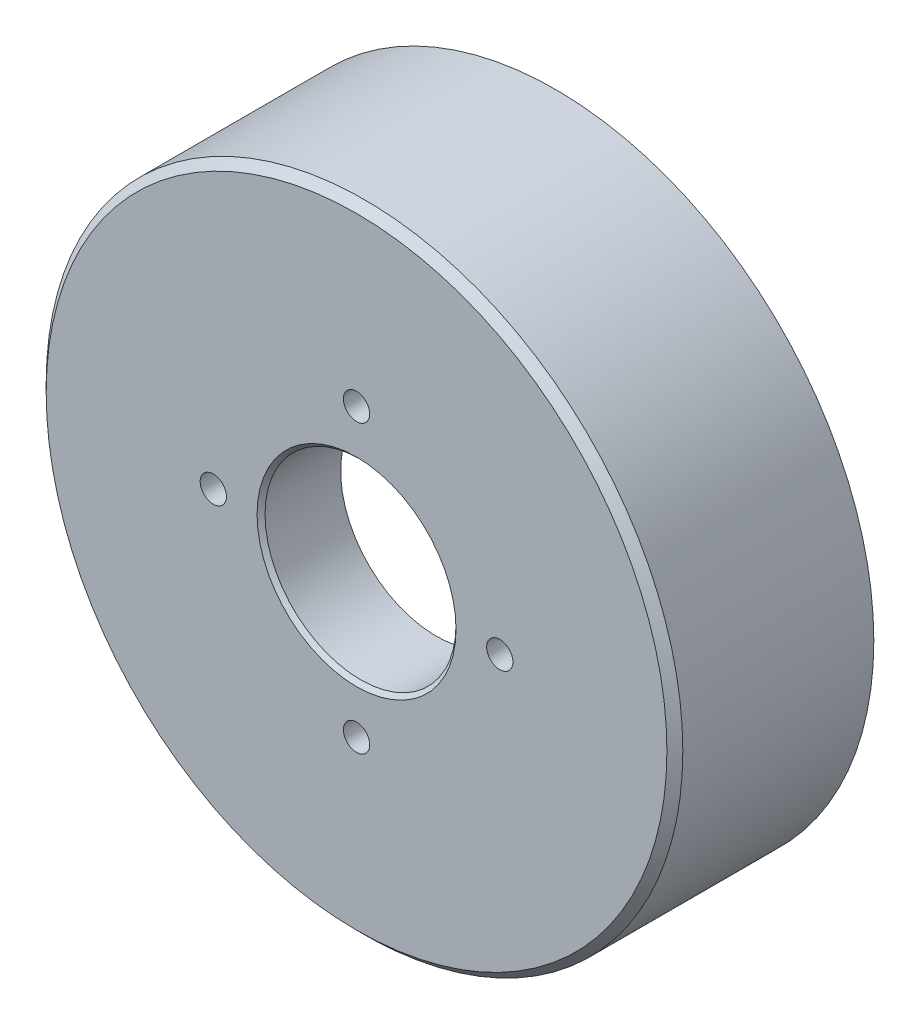
from build123d import *

# Parameters (mm, degrees)
CHAMFER1_SIZE      = 1
SKETCH9_R          = 12
CUT_EXTRUDE1_DEPTH = 62.846584384
M4_TAPPED_HOLE1_D  = 3.3
CHAMFER2_SIZE      = 0.5


with BuildPart() as part:
    # Sketch8 → Revolve2 (revolve)
    with BuildSketch(Plane(origin=(0, 0, 0), x_dir=(0, 0, -1), z_dir=(1, 0, 0)), mode=Mode.PRIVATE) as revolve2_sk:
        Polygon((0, 0), (0, 40), (25, 40), (25, 35), (10, 35), (10, 0), align=None)
    revolve(revolve2_sk.sketch.rotate(Axis((0, 0, 0), (0, 0, -1)), 90), axis=Axis((0, 0, 0), (0, 0, -1)))

    # Chamfer1
    chamfer1_edges = [part.edges().sort_by_distance(p)[0] for p in [
        (-40, 0, 0),
    ]]
    chamfer(chamfer1_edges, length=CHAMFER1_SIZE)

    # Sketch9 → Cut-Extrude1 (cut, through all)
    with BuildSketch(Plane.XY):
        Circle(SKETCH9_R)
    extrude(amount=-CUT_EXTRUDE1_DEPTH, mode=Mode.SUBTRACT)

    # M4 Tapped Hole1 (through all)
    with Locations(Plane(origin=(0, 18, 0), x_dir=(1, 0, 0), z_dir=(0, 0, 1))):
        with Locations((0, 0), (-18, -18), (18, -18), (0, -36)):
            Hole(M4_TAPPED_HOLE1_D / 2)

    # Chamfer2
    chamfer2_edges = [part.edges().sort_by_distance(p)[0] for p in [
        (-12, 0, 0),
    ]]
    chamfer(chamfer2_edges, length=CHAMFER2_SIZE)


solid = part.part
